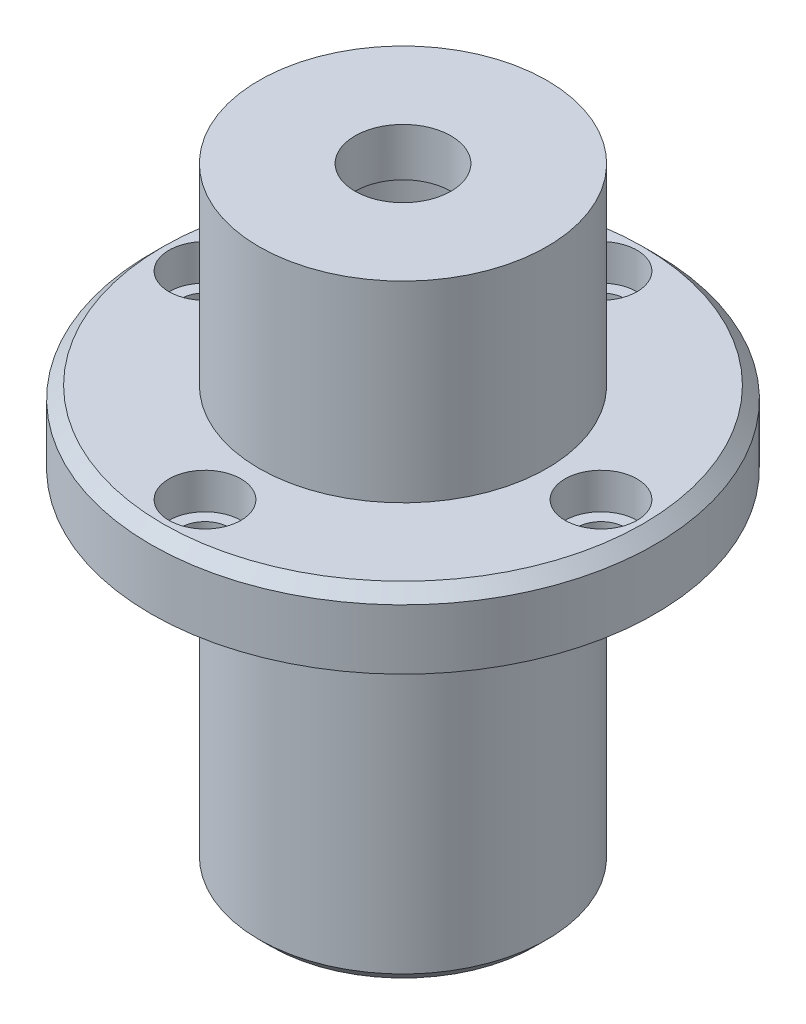
SolidWorks part; units mm, degrees
material "S45C"
ref_plane "Front Plane" through (0, 0, 0) normal (0, 0, 1) x (1, 0, 0)
ref_plane "Top Plane" through (0, 0, 0) normal (0, 1, 0) x (1, 0, 0)
ref_plane "Right Plane" through (0, 0, 0) normal (1, 0, 0) x (0, 0, -1)
sketch "Sketch1" plane through (0, 0, 0) normal (0, 1, 0) x (1, 0, 0)
  circle A0 centre (0, 0) radius 12
  circle A1 centre (0, 0) radius 4
  dimension "D1" = 8
  dimension "D2" = 24
extrude "Boss-Extrude1" add sketch "Sketch1" along normal blind 51
sketch "Sketch2" plane through (0, 0, 0) normal (0, -1, 0) x (1, 0, 0)
  circle A0 centre (0, 0) radius 8
  dimension "D1" = 16
extrude "Cut-Extrude1" cut sketch "Sketch2" against normal blind 47
ref_plane "Plane1" through (0, 35, 0) normal (0, 1, 0) x (-1, 0, 0)
sketch "Sketch3" plane through (0, 35, 0) normal (0, 1, 0) x (-1, 0, 0)
  circle A0 centre (0, 0) radius 21
  circle A1 centre (0, 0) radius 12
  circle A2 centre (0, 0) radius 12
  dimension "D2" = 42
  dimension "D1" = 0
extrude "Boss-Extrude2" add sketch "Sketch3" against normal blind 6
sketch "Sketch4" plane through (0, 35, 0) normal (0, 1, 0) x (1, 0, 0)
  circle A0 centre (0, 16.5) radius 2
  dimension "D2" = 4
  dimension "D1" = 16.5
extrude "Cut-Extrude2" cut sketch "Sketch4" against normal blind 6
sketch "Sketch5" plane through (0, 35, 0) normal (0, 1, 0) x (1, 0, 0)
  circle A0 centre (0, 16.5) radius 3
  dimension "D1" = 6
extrude "Cut-Extrude3" cut sketch "Sketch5" against normal blind 3
pattern_circular "CirPattern1" count 4 over 360 about axis through (0, 0, 0) along (0, 1, 0) of "Cut-Extrude3", "Cut-Extrude2"
chamfer "Chamfer1" distance 1 angle 45 2 edges at (0, 0, 12) (0, 35, 21)
